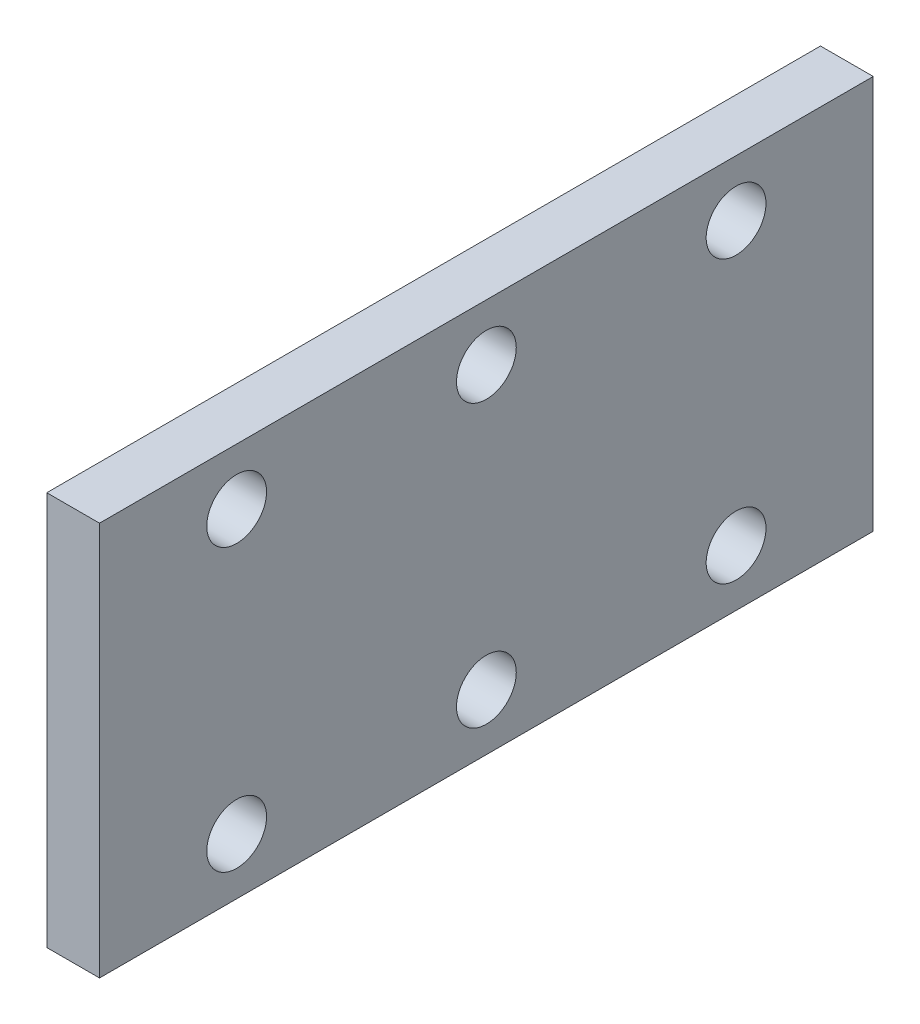
SolidWorks part; units mm, degrees
ref_plane "Front Plane" through (0, 0, 0) normal (0, 0, 1) x (1, 0, 0)
ref_plane "Top Plane" through (0, 0, 0) normal (0, 1, 0) x (1, 0, 0)
ref_plane "Right Plane" through (0, 0, 0) normal (1, 0, 0) x (0, 0, -1)
other "Configuration Table"
sketch "Sketch1" plane through (0, 0, 0) normal (0, 0, 1) x (1, 0, 0)
  line L0 (0, 0) -> (201.2265, 0) construction
  line L2 (75, 56) -> (60, 56)
  line L3 (75, 56) -> (75, -56)
  line L4 (75, -56) -> (60, -56)
  line L5 (60, 56) -> (60, 13)
  line L6 (75, 56) -> (60, -56) construction
  line L7 (75, -56) -> (60, 56) construction
  line L8 (43.0813, -13) -> (60, -13)
  line L10 (60, -13) -> (60, -56)
  line L11 (43.0813, 13) -> (60, 13)
  circle A0 centre (0, 0) radius 40
  arc A1 (43.0813, 13) -> (43.0813, -13) centre (0, 0) ccw
  point P5 (67.5, 0)
  dimension "D1" = 80
  dimension "D2" = 90
  dimension "D5" = 60
  dimension "D3" = 15
  dimension "D4" = 112
extrude "Boss-Extrude1" add sketch "Sketch1" along normal blind 220
sketch "Sketch2" plane through (75, 0, 0) normal (1, 0, 0) x (0, 0, -1)
  line L0 (0, -56) -> (0, 56) construction
  line L1 (-181, -40) -> (-39, -40) construction
  line L2 (-181, -40) -> (-181, 40) construction
  line L3 (-181, 40) -> (-39, 40) construction
  line L4 (-39, -40) -> (-39, 40) construction
  line L5 (-181, -40) -> (-39, 40) construction
  line L6 (-181, 40) -> (-39, -40) construction
  line L7 (-220, -56) -> (-220, 56) construction
  circle A0 centre (-181, -40) radius 8.5
  circle A1 centre (-181, 40) radius 8.5
  circle A2 centre (-110, 40) radius 8.5
  circle A3 centre (-110, -40) radius 8.5
  circle A4 centre (-39, -40) radius 8.5
  circle A5 centre (-39, 40) radius 8.5
  point P0 (-110, 0)
  point P7 (0, 0)
  dimension "D5" = 17
  dimension "D1" = 80
  dimension "D2" = 40
  dimension "D3" = 39
  dimension "D4" = 39
extrude "Cut-Extrude1" cut sketch "Sketch2" against normal up to next
sketch "Sketch3" plane through (0, 0, 0) normal (0, 1, 0) x (1, 0, 0)
  line L0 (40, 0) -> (-40, 0) construction
  line L1 (-45, -220) -> (43.0813, -220) construction
  circle A0 centre (0, -10) radius 2.5
  circle A1 centre (-0.9593, -210) radius 2.5
  dimension "D1" = 5
  dimension "D2" = 10
  dimension "D3" = 5
  dimension "D4" = 10
extrude "Cut-Extrude2" cut sketch "Sketch3" against normal up to next
sketch "Sketch4" plane through (0, 0, 220) normal (0, 0, 1) x (1, 0, 0)
  line L1 (60, -56) -> (-66.8719, -56)
  line L2 (60, -56) -> (60, 111.2453)
  line L3 (60, 111.2453) -> (-66.8719, 111.2453)
  line L4 (-66.8719, -56) -> (-66.8719, 111.2453)
extrude "Cut-Extrude3" cut sketch "Sketch4" against normal up to next
